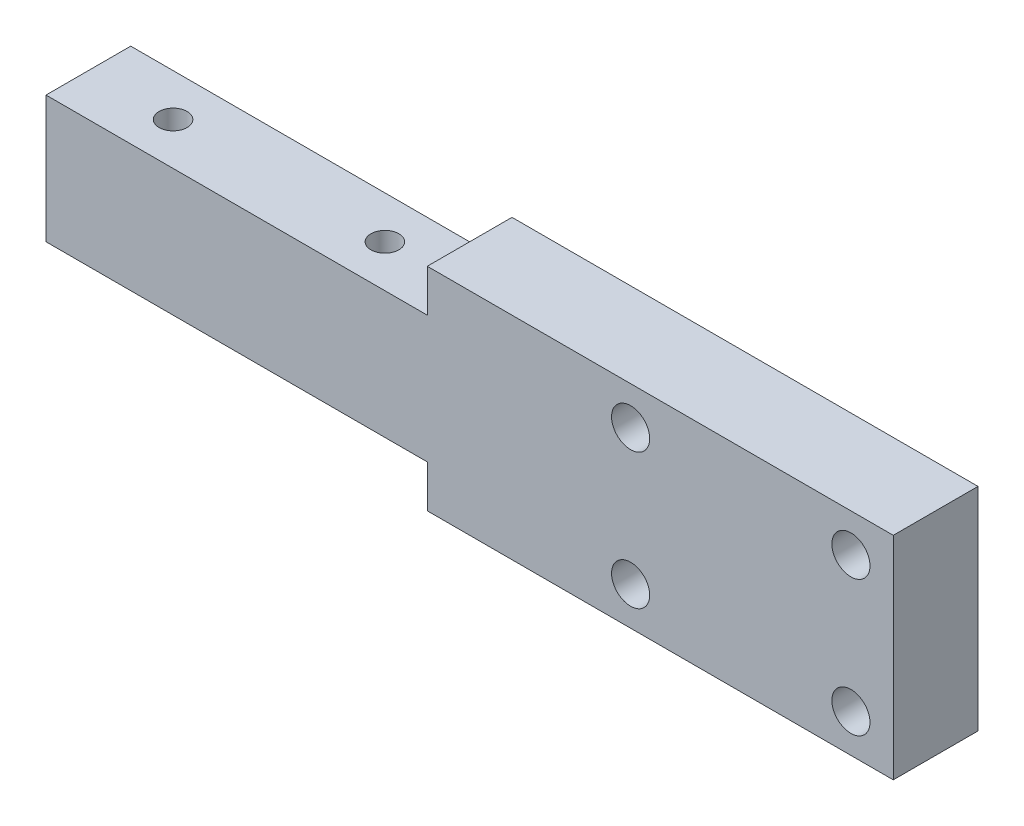
SolidWorks part; units mm, degrees
ref_plane "Front Plane" through (0, 0, 0) normal (0, 0, 1) x (1, 0, 0)
ref_plane "Top Plane" through (0, 0, 0) normal (0, 1, 0) x (1, 0, 0)
ref_plane "Right Plane" through (0, 0, 0) normal (1, 0, 0) x (0, 0, -1)
sketch "Sketch1" plane through (0, 0, 0) normal (0, 0, 1) x (1, 0, 0)
  line L1 (-50, 12.5) -> (50, 12.5)
  line L2 (-50, 12.5) -> (-50, -12.5)
  line L3 (-50, -12.5) -> (50, -12.5)
  line L4 (50, 12.5) -> (50, -12.5)
  line L5 (-50, 12.5) -> (50, -12.5) construction
  line L6 (-50, -12.5) -> (50, 12.5) construction
  point P0 (0, 0)
  dimension "D1" = 100
  dimension "D2" = 25
extrude "Boss-Extrude1" add sketch "Sketch1" along normal blind 10
sketch "Sketch2" plane through (0, 0, 0) normal (0, 0, -1) x (-1, 0, 0)
  line L1 (0, 0) -> (56.4059, 0) construction
  line L3 (50, 12.5) -> (5, 12.5)
  line L5 (50, 12.5) -> (50, 7.5)
  line L6 (50, 7.5) -> (5, 7.5)
  line L7 (5, 12.5) -> (5, 7.5)
  line L8 (5, -12.5) -> (5, -7.5)
  line L9 (50, -7.5) -> (5, -7.5)
  line L10 (50, -12.5) -> (50, -7.5)
  line L11 (50, -12.5) -> (5, -12.5)
  dimension "D1" = 45
  dimension "D2" = 5
extrude "Cut-Extrude1" cut sketch "Sketch2" against normal through all both and the other way through all
hole_wizard "Hole for socket head cap screw, type1" positions "Sketch4" profile "Sketch3" counterbore size "M4" standard "GB"
sketch "Sketch4" plane through (0, 0, 0) normal (0, 0, -1) x (-1, 0, 0)
  point P1 (-19, -8)
  point P5 (-19, 8)
  point P9 (-45, 8)
  point P13 (-45, -8)
  dimension "D1" = 26
  dimension "D2" = 19
  dimension "D3" = 8
  dimension "D4" = 8
sketch "Sketch3" plane through (19, -8, 0) normal (1, 0, 0) x (0, 1, 0)
  line L0 (0, 0) -> (0, 10)
  line L1 (0, 10) -> (2.25, 10)
  line L3 (2.25, 10) -> (2.25, 4.6)
  line L4 (2.25, 4.6) -> (4, 4.6)
  line L5 (4, 4.6) -> (4, 0)
  line L7 (4, 0) -> (0, 0)
  line L11 (0, -6.35) -> (0, 107.95) construction
  dimension "通孔孔直径" = 4.5
  dimension "通孔孔深度" = 10
  dimension "柱形沉头孔直径" = 8
  dimension "柱形沉头孔深度" = 4.6
hole_wizard "M4 Tapped Hole1" positions "Sketch6" profile "Sketch5" tap size "M4" standard "GB" end condition through all
sketch "Sketch6" plane through (0, 7.5, 0) normal (0, 1, 0) x (1, 0, 0)
  point P1 (-15, -5)
  point P5 (-40, -5)
  dimension "D1" = 25
  dimension "D2" = 15
  dimension "D3" = 5
sketch "Sketch5" plane through (-15, 7.5, 5) normal (1, 0, 0) x (0, 0, 1)
  line L0 (0, 0) -> (0, 20)
  line L1 (0, 20) -> (1.65, 20)
  line L2 (1.65, 20) -> (1.65, 0)
  line L5 (1.65, 0) -> (0, 0)
  line L11 (0, -6.35) -> (0, 107.95) construction
  dimension "通孔螺纹孔钻头直径" = 3.3
  dimension "通孔螺纹孔钻头深度" = 20
cosmetic thread "Cosmetic Thread1"
cosmetic thread "Cosmetic Thread2"
